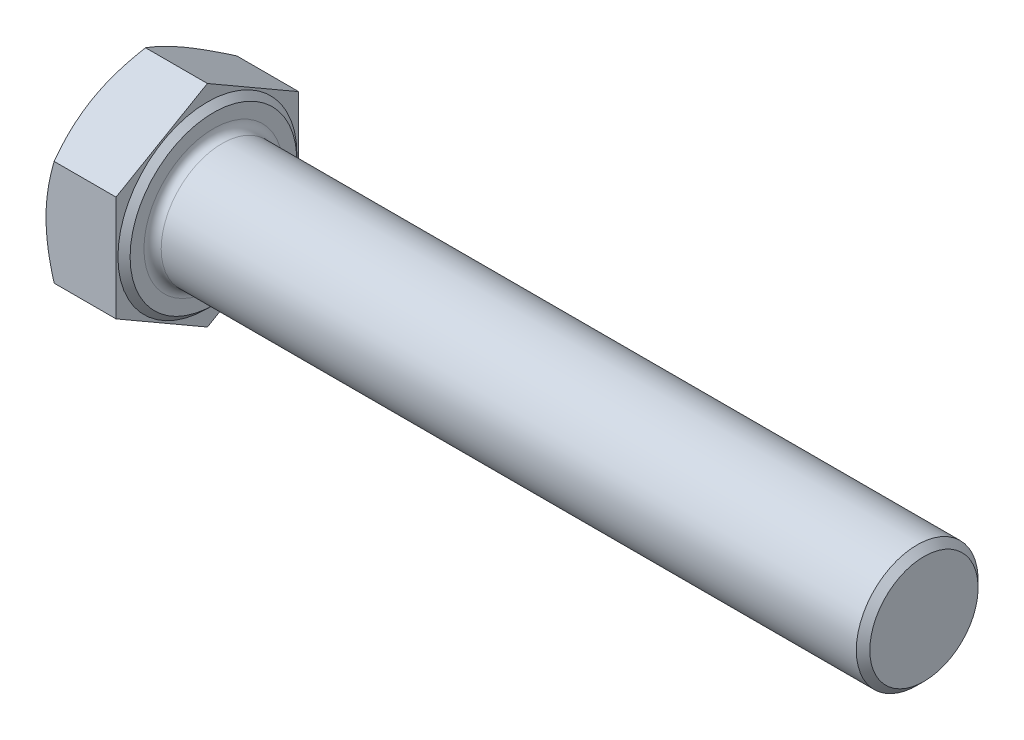
SolidWorks part; units mm, degrees
material "Q235"
ref_plane "Front Plane" through (0, 0, 0) normal (0, 0, 1) x (1, 0, 0)
ref_plane "Top Plane" through (0, 0, 0) normal (0, 1, 0) x (1, 0, 0)
ref_plane "Right Plane" through (0, 0, 0) normal (1, 0, 0) x (0, 0, -1)
sketch "Sketch1" plane through (0, 0, 0) normal (0, 0, 1) x (1, 0, 0)
  line L0 (0, 0) -> (77.5, 0) construction
  line L1 (0, 0) -> (0, 10.015)
  line L2 (0, 10.015) -> (7.5, 10.015)
  line L3 (7.5, 10.015) -> (7.5, 0)
  line L4 (7.5, 6) -> (77.5, 6)
  line L5 (77.5, 6) -> (77.5, 0)
  line L6 (0, 9) -> (0.586, 10.015)
  line L7 (74, 6) -> (74, 0)
  line L8 (12.8, 6) -> (12.8, 0)
  line L9 (7.5, 5.4317) -> (77.5, 5.4317)
  line L10 (77.5, 5.0528) -> (7.5, 5.0528)
  line L11 (6.9, 8.815) -> (7.5, 8.215)
  line L12 (6.9, 10.015) -> (6.9, 0)
  line L13 (7.4, 8.315) -> (7.4, 0) construction
  arc A0 (7.5, 6.85) -> (8.35, 6) centre (8.35, 6.85) ccw
  point P12 (75.75, 0)
  point P13 (2.38, 10.015)
  point P14 (7.5, 6.85)
  point P24 (7.5, 8.315)
  dimension "D1" = 0.1
  dimension "r" = 0.85
  dimension "k" = 7.5
  dimension "D2" = 45
  dimension "β" = 30
  dimension "e" = 20.03
  dimension "s" = 18
  dimension "d" = 12
  dimension "l" = 70
  dimension "D52" = 3.5
  dimension "P" = 1.75
  dimension "kw" = 5.12
  dimension "da" = 13.7
  dimension "a" = 5.3
  dimension "ds" = 10.8634
  dimension "D61" = 10.1056
  dimension "dw" = 16.63
  dimension "c" = 0.6
sketch "Sketch2" plane through (0, 0, 0) normal (1, 0, 0) x (0, 0, -1)
  line L1 (0, 10.3923) -> (-9, 5.1962)
  line L2 (-9, 5.1962) -> (-9, -5.1962)
  line L3 (-9, -5.1962) -> (0, -10.3923)
  line L4 (0, -10.3923) -> (9, -5.1962)
  line L5 (9, -5.1962) -> (9, 5.1962)
  line L6 (9, 5.1962) -> (0, 10.3923)
  circle A0 centre (0, 0) radius 9 construction
sketch "Sketch3" plane through (0, 0, 0) normal (1, 0, 0) x (0, 0, -1)
  line L0 (9, 5.1962) -> (0, 10.3923) construction
  line L1 (0, 10.3923) -> (-9, 5.1962) construction
  line L2 (-9, 5.1962) -> (-9, -5.1962) construction
  line L3 (9, -5.1962) -> (9, 5.1962) construction
  line L4 (0, -10.3923) -> (9, -5.1962) construction
  line L5 (-9, -5.1962) -> (0, -10.3923) construction
  line L6 (9, 5.1962) -> (0, 10.3923)
  line L7 (0, 10.3923) -> (-9, 5.1962)
  line L8 (-9, 5.1962) -> (-9, -5.1962)
  line L9 (9, -5.1962) -> (9, 5.1962)
  line L10 (0, -10.3923) -> (9, -5.1962)
  line L11 (-9, -5.1962) -> (0, -10.3923)
extrude "Boss-Extrude1" add sketch "Sketch3" along normal up to vertex (7.5 mm away) up to point (7.5, 10.015, 0)
sketch "Sketch4" plane through (0, 0, 0) normal (-1, 0, 0) x (0, 0, 1)
  circle A0 centre (0, 0) radius 9 construction
  circle A1 centre (0, 0) radius 9
  circle A2 centre (0, 0) radius 20.03
  dimension "D1" = 40.06
extrude "Cut-Extrude1" cut sketch "Sketch4" against normal blind 0.9375 draft 60
sketch "Sketch5" plane through (0, 0, 0) normal (0, 0, 1) x (1, 0, 0)
  line L0 (7.5, 6) -> (77.5, 6) construction
  line L1 (77.5, 6) -> (77.5, 0) construction
  line L2 (0, 0) -> (77.5, 0) construction
  line L3 (8.35, 6) -> (77.5, 6)
  line L4 (77.5, 6) -> (77.5, 0)
  line L5 (7.5, 0) -> (77.5, 0)
  line L6 (7.5, 6.85) -> (7.5, 0)
  arc A0 (7.5, 6.85) -> (8.35, 6) centre (8.35, 6.85) ccw construction
  arc A1 (7.5, 6.85) -> (8.35, 6) centre (8.35, 6.85) ccw
revolve "Revolve1" add sketch "Sketch5" angle 360 about L5
cosmetic thread "Cosmetic Thread2" parameters "D1"=64.7, "D2"=10.1056
chamfer "Chamfer2" distance 0.6667 angle 45 1 edges at (77.5, 0, 6)
sketch "Sketch7" plane through (0, 0, 0) normal (0, 0, 1) x (1, 0, 0)
  line L0 (7.5, 8.215) -> (6.9, 8.815)
  line L1 (6.9, 8.815) -> (6.9, 20.03)
  line L2 (6.9, 20.03) -> (7.5, 20.03)
  line L3 (7.5, 20.03) -> (7.5, 8.215)
  line L4 (0, 0) -> (77.5, 0) construction
  line L5 (0, 0) -> (77.5, 0) construction
  dimension "D1" = 40.06
revolve "Cut-Revolve1" cut sketch "Sketch7" angle 360 mid plane about L5
sketch "Sketch6" [suppressed] plane through (0, 0, 0) normal (0, 0, 1) x (1, 0, 0)
  line L0 (9.3, 0) -> (9.3, 4) construction
  line L1 (9.3, 4) -> (75.3, 4)
  line L2 (75.3, 4) -> (75.3, 0)
  line L3 (9.3, 4) -> (5.9719, 3.5984)
  line L5 (5.3, 3.5941) -> (75.3, 3.5941) construction
  line L6 (5.3, 7.19) -> (5.3, 0) construction
  line L7 (5.3, 4.1941) -> (5.3, 0)
  line L8 (5.3, 0) -> (75.3, 0)
  arc A0 (5.9719, 3.5984) -> (5.3, 4.1941) centre (5.9, 4.1941) cw
  arc A1 (5.3, 4.6) -> (5.9, 4) centre (5.9, 4.6) ccw construction
revolve "Revolve2" add sketch "Sketch6" angle 360 about L8
cosmetic thread "Cosmetic Thread1" [suppressed] parameters "D1"=64.7, "D2"=10.1056
chamfer "Chamfer1" [suppressed] distance 0.6667 angle 45
sketch "Sketch8" [suppressed] plane through (0, 0, 0) normal (0, 0, 1) x (1, 0, 0)
  line L0 (5.3, 5.715) -> (4.7, 6.315)
  line L1 (4.7, 6.315) -> (4.7, 14.38)
  line L2 (4.7, 14.38) -> (5.3, 14.38)
  line L3 (5.3, 14.38) -> (5.3, 5.715)
  line L4 (0, 0) -> (75.3, 0) construction
  line L5 (0, 0) -> (75.3, 0) construction
  dimension "D1" = 40.06
revolve "Cut-Revolve2" [suppressed] cut sketch "Sketch8" angle 360 mid plane about L5
